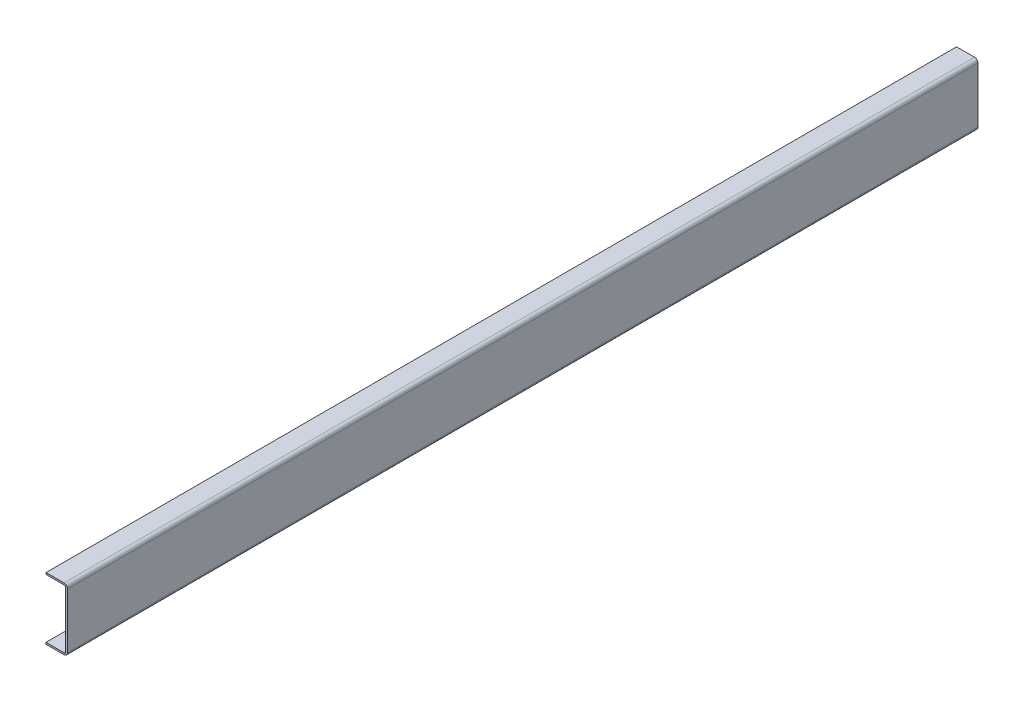
SolidWorks part; units mm, degrees
ref_plane "Front Plane" through (0, 0, 0) normal (0, 0, 1) x (1, 0, 0)
ref_plane "Top Plane" through (0, 0, 0) normal (0, 1, 0) x (1, 0, 0)
ref_plane "Right Plane" through (0, 0, 0) normal (1, 0, 0) x (0, 0, -1)
other "Configuration Table"
sketch "Sketch1" plane through (0, 0, 0) normal (0, 0, 1) x (1, 0, 0)
  line L0 (-50, -72.5) -> (-8, -72.5)
  line L1 (0, -64.5) -> (0, 64.5)
  line L2 (-8, 72.5) -> (-50, 72.5)
  line L3 (-50, 72.5) -> (-50, 68.5)
  line L4 (-50, 68.5) -> (-8, 68.5)
  line L5 (-4, 64.5) -> (-4, -64.5)
  line L6 (-8, -68.5) -> (-50, -68.5)
  line L7 (-50, -68.5) -> (-50, -72.5)
  arc A0 (-8, -72.5) -> (0, -64.5) centre (-8, -64.5) ccw
  arc A1 (0, 64.5) -> (-8, 72.5) centre (-8, 64.5) ccw
  arc A2 (-4, 64.5) -> (-8, 68.5) centre (-8, 64.5) ccw
  arc A3 (-8, -68.5) -> (-4, -64.5) centre (-8, -64.5) ccw
  dimension "D1" = 8
  dimension "D2" = 4
  dimension "D3" = 50
  dimension "D4" = 68.5
  dimension "D5" = 68.5
extrude "Boss-Extrude1" add sketch "Sketch1" along normal mid plane 2124
